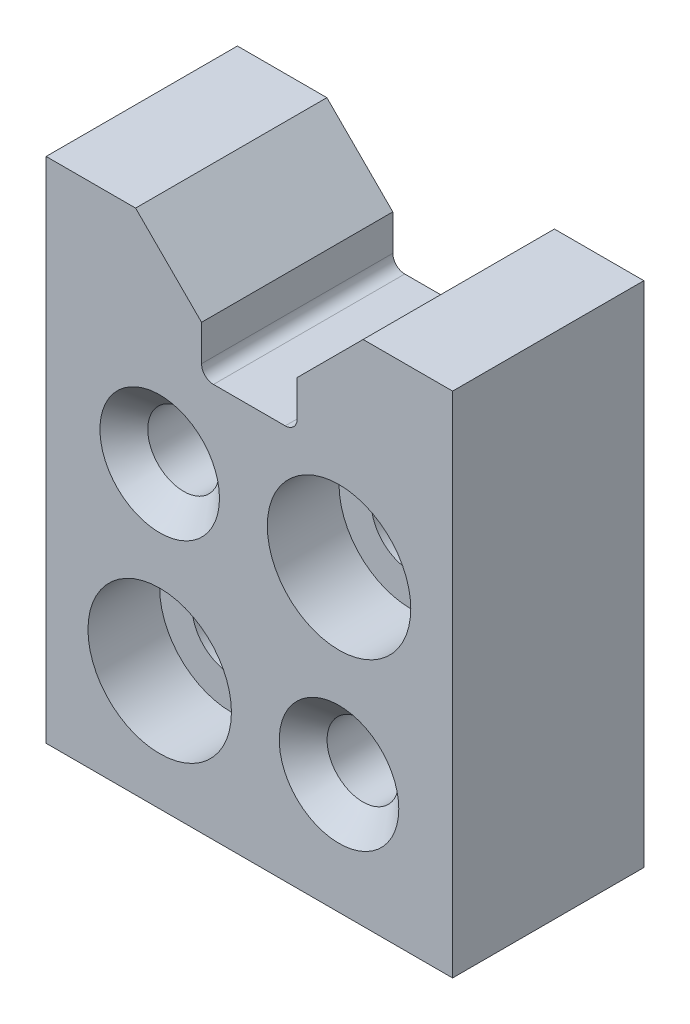
SolidWorks part; units mm, degrees
extrude "Base-Extrude" add sketch "Sketch1" along normal blind 16
sketch "Sketch1" plane through (0, 0, 0) normal (0, 0, 1) x (1, 0, 0)
  line L0 (0, 70) -> (0, -60) construction
  line L1 (-17, 50.8486) -> (17, 50.8486)
  line L2 (-17, 50.8486) -> (-17, 5.8486)
  line L3 (-17, 5.8486) -> (17, 5.8486)
  line L4 (17, 50.8486) -> (17, 5.8486)
  dimension "D1" = 17
  dimension "L" = 45
  dimension "B" = 34
material "镍"
ref_plane "Front view" through (0, 0, 0) normal (0, 0, 1) x (1, 0, 0)
ref_plane "Top view" through (0, 0, 0) normal (0, 1, 0) x (1, 0, 0)
ref_plane "Right view" through (0, 0, 0) normal (1, 0, 0) x (0, 0, -1)
sketch "Sketch2" plane through (0, 0, 16) normal (0, 0, 1) x (1, 0, 0)
  line L0 (0, 60) -> (0, -50) construction
  line L1 (-4, 38.8486) -> (4, 38.8486)
  line L2 (-4, 38.8486) -> (-4, 42.8486)
  line L3 (-12, 50.8486) -> (12, 50.8486)
  line L4 (4, 38.8486) -> (4, 42.8486)
  line L8 (-12, 50.8486) -> (-4, 42.8486)
  line L9 (12, 50.8486) -> (4, 42.8486)
  point P9 (0, 50.8486)
extrude "Cut-Extrude1" cut sketch "Sketch2" against normal through all
sketch "Sketch3" plane through (0, 0, 16) normal (0, 0, 1) x (1, 0, 0)
  line L0 (0, 70) -> (0, -60) construction
  line L1 (-7.5, 47.938) -> (-7.5, -45.8462) construction
  line L2 (7.5, 47.938) -> (7.5, -45.8462) construction
  line L3 (-50, 15.8486) -> (60, 15.8486) construction
  line L4 (-60, 30.8486) -> (60, 30.8486) construction
  line L5 (-17, 5.8486) -> (17, 5.8486) construction
  circle A0 centre (-7.5, 30.8486) radius 3
  circle A1 centre (7.5, 15.8486) radius 3
  point P13 (-7.5, 30.8486)
  point P14 (-7.5, 15.8486)
  point P15 (7.5, 30.8486)
  point P16 (7.5, 15.8486)
hole_wizard "CBORE for M5 Hex Head Screw1" positions "Sketch10" profile "Sketch9" counterbore size "M5" standard "ISO" end condition through all
sketch "Sketch10" plane through (0, 0, 16) normal (0, 0, 1) x (1, 0, 0)
  line L0 (-17, 5.8486) -> (17, 5.8486) construction
  point P0 (7.5, 30.8486)
sketch "Sketch9" plane through (7.5, 30.8486, 16) normal (1, 0, 0) x (0, -1, 0)
  line L0 (0, 0) -> (0, 16)
  line L1 (0, 16) -> (3.3, 16)
  line L3 (3.3, 16) -> (3.3, 6)
  line L4 (3.3, 6) -> (6, 6)
  line L5 (6, 6) -> (6, 0)
  line L7 (6, 0) -> (0, 0)
  line L11 (0, -6.35) -> (0, 107.95) construction
extrude "Cut-Extrude4" cut sketch "Sketch3" against normal blind 25
chamfer "Chamfer3" distance 2 angle 45 2 edges at (-4.5, 30.8486, 16) (10.5, 15.8486, 16)
chamfer "Chamfer4" distance 2 angle 45 2 edges at (-4.5, 30.8486, 0) (10.5, 15.8486, 0)
hole_wizard "CBORE for M5 Hex Head Screw2" positions "Sketch12" profile "Sketch11" counterbore size "M5" standard "ISO" end condition through all
sketch "Sketch12" plane through (0, 0, 16) normal (0, 0, 1) x (1, 0, 0)
  line L1 (-17, 5.8486) -> (17, 5.8486) construction
  point P0 (-7.5, 15.8486)
sketch "Sketch11" plane through (-7.5, 15.8486, 16) normal (1, 0, 0) x (0, -1, 0)
  line L0 (0, 0) -> (0, 16)
  line L1 (0, 16) -> (3.3, 16)
  line L3 (3.3, 16) -> (3.3, 6)
  line L4 (3.3, 6) -> (6, 6)
  line L5 (6, 6) -> (6, 0)
  line L7 (6, 0) -> (0, 0)
  line L11 (0, -6.35) -> (0, 107.95) construction
fillet "Fillet1" radius 1 1 edges at (-4, 38.8486, 8)
fillet "Fillet2" radius 1 1 edges at (4, 38.8486, 8)
sketch "Sketch13" plane through (0, 0, 16) normal (0, 0, 1) x (1, 0, 0)
  line L1 (-19.1251, 54.0346) -> (18.6707, 54.0346)
  line L2 (-19.1251, 54.0346) -> (-19.1251, 48.3652)
  line L3 (-19.1251, 48.3652) -> (18.6707, 48.3652)
  line L4 (18.6707, 54.0346) -> (18.6707, 48.3652)
extrude "Cut-Extrude5" cut sketch "Sketch13" against normal through all
equation "\"D3@Sketch2\" = \"N@Sketch2\" / 2"
equation "\"D4@Sketch2\" = \"b1@Sketch2\" / 2"
equation "\"柱形沉头孔直径@Sketch11\" = \"d2@Sketch9\""
equation "\"柱形沉头孔深度@Sketch11\" = \"h1@Sketch9\""
equation "\"通孔孔直径@Sketch11\" = \"d1@Sketch9\""
equation "\"D1@Fillet1\" = \"r@Fillet2\""
equation "\"D2@Sketch3\" = \"d3@Sketch3\""
equation "\"D1@Sketch1\"  = \"B@Sketch1\" /  2"
equation "\"D2@Sketch12\" = \"l1@Sketch3\""
equation "\"D1@Sketch12\" = \"D1@Sketch3\""
equation "\"D1@Sketch10\" = \"D1@Sketch3\""
equation "\"D2@Sketch10\" = \"A1@Sketch3\" + \"l1@Sketch3\""
equation "\"D2@Sketch2\" = \"D1@Sketch2\""
